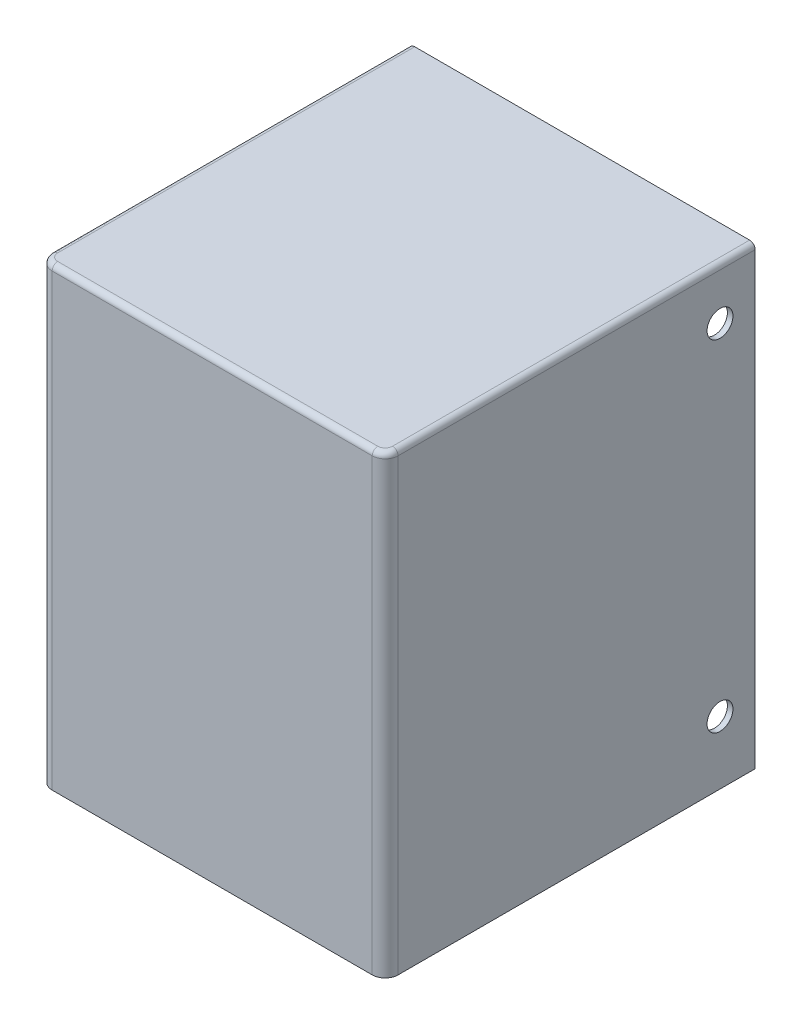
from build123d import *

# Parameters (mm, degrees)
SKETCH_1_W          = 93.5
SKETCH_1_H          = 123
SKETCH_1_W_2        = 90.5
SKETCH_1_H_2        = 120
EXTRUDE_1_DEPTH     = 100
SKETCH_2_W          = 93.5
SKETCH_2_H          = 123
EXTRUDE_2_DEPTH     = 1.5
SKETCH_3_W          = 90.5
SKETCH_3_H          = 98.5
CUT_EXTRUDE_1_DEPTH = 3
SKETCH_4_R          = 3.5
CUT_EXTRUDE_2_DEPTH = 151.081644447
FILLET_1_R          = 2
FILLET_2_R          = 3.5
FILLET_3_R          = 1
FILLET_4_R          = 1.5


with BuildPart() as part:
    # 草图1 → 凸台-拉伸1 (new body)
    with BuildSketch(Plane.XY):
        Rectangle(SKETCH_1_W, SKETCH_1_H)
        Rectangle(SKETCH_1_W_2, SKETCH_1_H_2, mode=Mode.SUBTRACT)
    extrude(amount=EXTRUDE_1_DEPTH)

    # 草图2 → 凸台-拉伸2 (add)
    with BuildSketch(Plane.XY.offset(100)):
        Rectangle(SKETCH_2_W, SKETCH_2_H)
    extrude(amount=-EXTRUDE_2_DEPTH)

    # 草图3 → 切除-拉伸1 (cut)
    with BuildSketch(Plane.XZ.offset(61.5)):
        with Locations((0, 49.25)):
            Rectangle(SKETCH_3_W, SKETCH_3_H)
    extrude(amount=-CUT_EXTRUDE_1_DEPTH, mode=Mode.SUBTRACT)

    # 草图4 → 切除-拉伸2 (cut, through all)
    with BuildSketch(Plane(origin=(46.75, 0, 0), x_dir=(0, 0, -1), z_dir=(1, 0, 0))):
        with Locations((-9.5, -44.5)):
            Circle(SKETCH_4_R)
        with Locations((-9.5, 47.5)):
            Circle(SKETCH_4_R)
    extrude(amount=-CUT_EXTRUDE_2_DEPTH, mode=Mode.SUBTRACT)

    # 圆角1
    fillet_1_edges = [part.edges().sort_by_distance(p)[0] for p in [
        (45.25, -0.75, 98.5),
        (-45.25, -0.75, 98.5),
    ]]
    fillet(fillet_1_edges, radius=FILLET_1_R)

    # 圆角2
    fillet_2_edges = [part.edges().sort_by_distance(p)[0] for p in [
        (-46.75, 0, 100),
        (46.75, 0, 100),
    ]]
    fillet(fillet_2_edges, radius=FILLET_2_R)

    # 圆角3
    fillet_3_edges = [part.edges().sort_by_distance(p)[0] for p in [
        (-45.25, 60, 48.25),
        (0, 60, 98.5),
        (45.25, 60, 48.25),
        (44.664213562, 60, 97.914213562),
        (-44.664213562, 60, 97.914213562),
    ]]
    fillet(fillet_3_edges, radius=FILLET_3_R)

    # 圆角4
    fillet_4_edges = [part.edges().sort_by_distance(p)[0] for p in [
        (46.75, 61.5, 48.25),
        (-46.75, 61.5, 48.25),
        (-45.724873734, 61.5, 98.974873734),
        (45.724873734, 61.5, 98.974873734),
        (0, 61.5, 100),
    ]]
    fillet(fillet_4_edges, radius=FILLET_4_R)


solid = part.part
